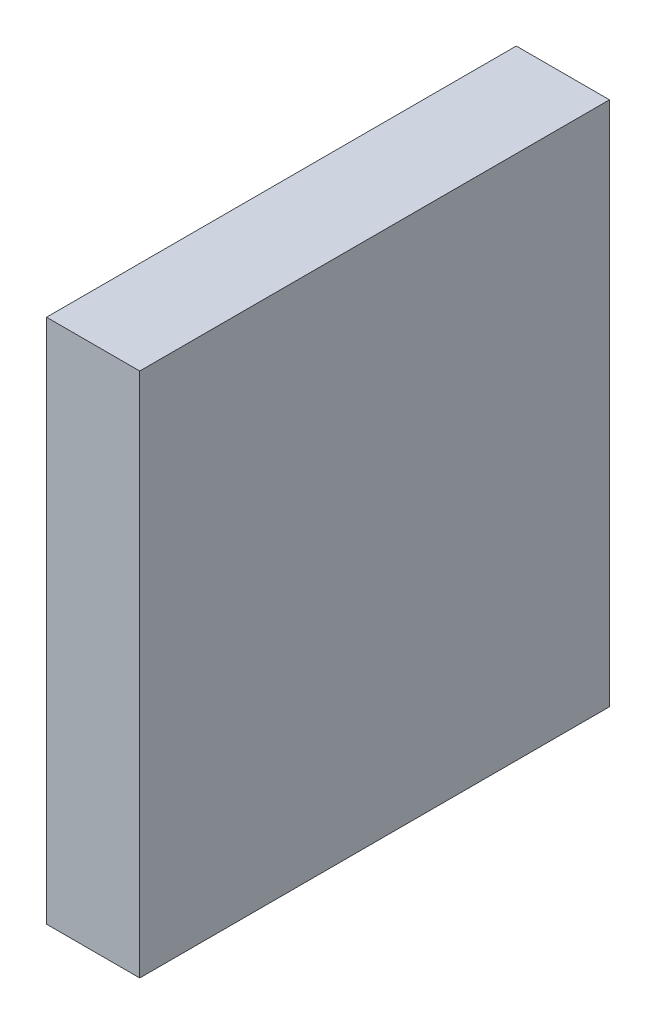
from build123d import *

# Parameters (mm, degrees)
SKETCH2_W           = 25
SKETCH2_H           = 126
BOSS_EXTRUDE1_DEPTH = 70.5


with BuildPart() as part:
    # Sketch2 → Boss-Extrude1 (new, symmetric)
    with BuildSketch(Plane(origin=(0, 0, 0), x_dir=(1, 0, 0), z_dir=(0, 1, 0))):
        Rectangle(SKETCH2_W, SKETCH2_H)
    extrude(amount=BOSS_EXTRUDE1_DEPTH, both=True)


solid = part.part
